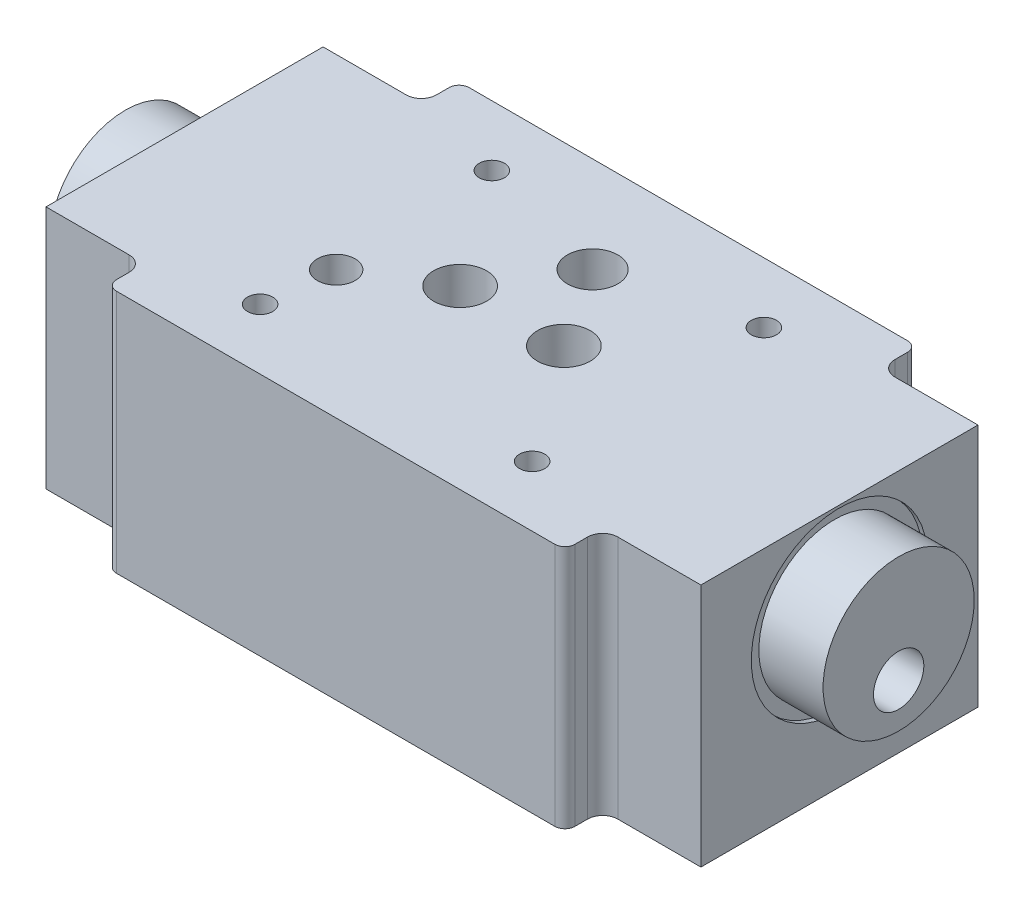
from build123d import *

# Parameters (mm, degrees)
BOSS_EXTRUDE_1_DEPTH = 24.25
SKETCH_2_R           = 17.5
CUT_EXTRUDE_3_DEPTH  = 1
SKETCH_3_R           = 15
BOSS_EXTRUDE_3_DEPTH = 76.75
SKETCH_4_R           = 5
SKETCH_4_R_2         = 5.25
SKETCH_4_R_3         = 3.75
CUT_EXTRUDE_1_DEPTH  = 98.302684958
M6_THREADED_HOLE_1_D = 5
SKETCH_5_R           = 5
CUT_EXTRUDE_2_DEPTH  = 160.2963041


with BuildPart() as part:
    # Sketch 1 → Boss-Extrude 1 (new, symmetric)
    with BuildSketch(Plane(origin=(0, 0, 0), x_dir=(1, 0, 0), z_dir=(0, 1, 0))):
        with BuildLine():
            Line((43.5, 35), (-43.5, 35))
            ThreePointArc((-43.5, 35), (-44.914213562, 34.414213562), (-45.5, 33))
            Line((-45.5, 33), (-45.5, 30.5))
            ThreePointArc((-45.5, 30.5), (-46.378679656, 28.378679656), (-48.5, 27.5))
            Line((-48.5, 27.5), (-65, 27.5))
            Line((-65, 27.5), (-65, -27.5))
            Line((-65, -27.5), (-48.5, -27.5))
            ThreePointArc((-48.5, -27.5), (-46.378679656, -28.378679656), (-45.5, -30.5))
            Line((-45.5, -30.5), (-45.5, -33))
            ThreePointArc((-45.5, -33), (-44.914213562, -34.414213562), (-43.5, -35))
            Line((-43.5, -35), (43.5, -35))
            ThreePointArc((43.5, -35), (44.914213562, -34.414213562), (45.5, -33))
            Line((45.5, -33), (45.5, -30.5))
            ThreePointArc((45.5, -30.5), (46.378679656, -28.378679656), (48.5, -27.5))
            Line((48.5, -27.5), (65, -27.5))
            Line((65, -27.5), (65, 27.5))
            Line((65, 27.5), (48.5, 27.5))
            ThreePointArc((48.5, 27.5), (46.378679656, 28.378679656), (45.5, 30.5))
            Line((45.5, 30.5), (45.5, 33))
            ThreePointArc((45.5, 33), (44.914213562, 34.414213562), (43.5, 35))
        make_face()
    extrude(amount=BOSS_EXTRUDE_1_DEPTH, both=True)

    # Sketch 2 → Cut-Extrude 3 (cut)
    with BuildSketch(Plane(origin=(65, 0, 0), x_dir=(0, 0, -1), z_dir=(1, 0, 0))):
        with Locations((0, 6.25)):
            Circle(SKETCH_2_R)
    cut_extrude_3 = extrude(amount=-CUT_EXTRUDE_3_DEPTH, mode=Mode.SUBTRACT)

    # Mirror 1: Cut-Extrude 3 across plane
    add(cut_extrude_3.mirror(Plane(origin=(0, 0, 0), x_dir=(0, 0, 1), z_dir=(1, 0, 0))), mode=Mode.SUBTRACT)

    # Sketch 3 → Boss-Extrude 3 (add, symmetric)
    with BuildSketch(Plane(origin=(0, 0, 0), x_dir=(0, 0, -1), z_dir=(1, 0, 0))):
        with Locations(Location((0, 6.25, 0), (0, 0, 180))):
            Circle(SKETCH_3_R)
    extrude(amount=BOSS_EXTRUDE_3_DEPTH, both=True)

    # Sketch 4 → Cut-Extrude 1 (cut, through all)
    with BuildSketch(Plane(origin=(0, 24.25, 0), x_dir=(1, 0, 0), z_dir=(0, 1, 0))):
        with Locations(Location((0, 16, 0), (0, 0, 270))):
            Circle(SKETCH_4_R)
        with Locations(Location((-10.3, 0, 0), (0, 0, 270))):
            Circle(SKETCH_4_R_2)
        with Locations(Location((-25.4, -9.5, 0), (0, 0, 270))):
            Circle(SKETCH_4_R_3)
        with Locations(Location((10.3, 0, 0), (0, 0, 270))):
            Circle(SKETCH_4_R_2)
    extrude(amount=-CUT_EXTRUDE_1_DEPTH, mode=Mode.SUBTRACT)

    # M6 threaded hole 1 (through all)
    with Locations(Plane(origin=(-27, 24.25, -23), x_dir=(0, 0, 1), z_dir=(0, 1, 0))):
        with Locations((0, 0), (0, 54), (46, 54), (46, 0)):
            Hole(M6_THREADED_HOLE_1_D / 2)

    # Sketch 5 → Cut-Extrude 2 (cut, through all)
    with BuildSketch(Plane(origin=(76.75, 0, 0), x_dir=(0, 0, -1), z_dir=(1, 0, 0))):
        Circle(SKETCH_5_R)
    extrude(amount=-CUT_EXTRUDE_2_DEPTH, mode=Mode.SUBTRACT)


solid = part.part
